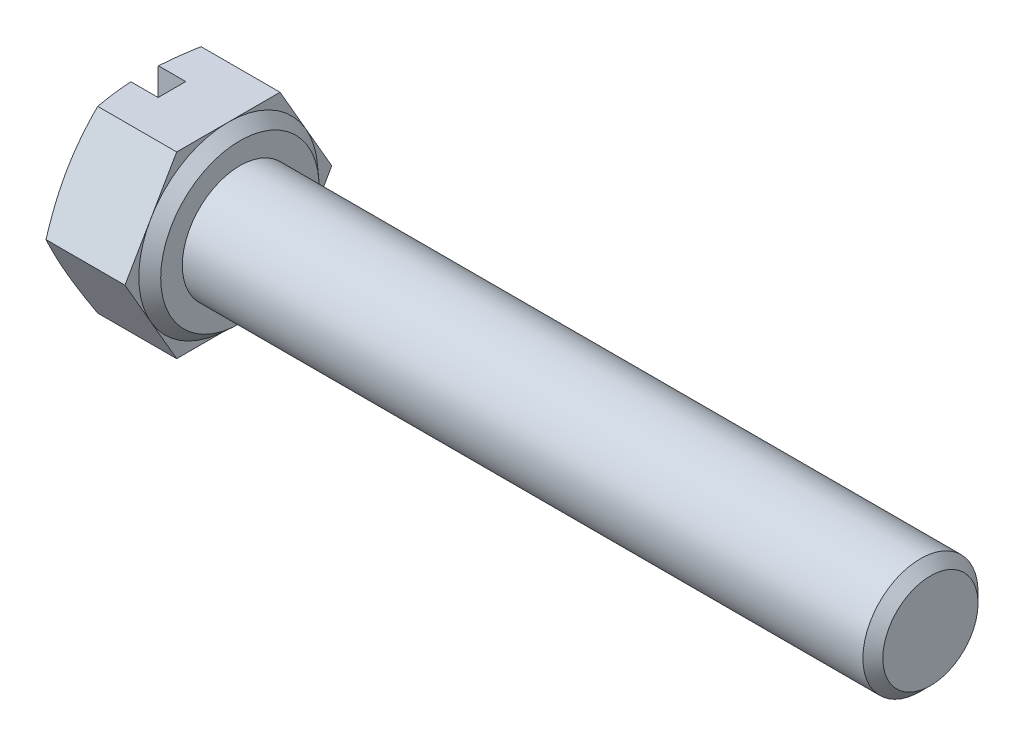
from build123d import *

# Parameters (mm, degrees)
BASEHEAD_DEPTH  = 3.65
SKETCH3_R       = 2.5
BASEBODY_DEPTH  = 30
CHAMFER1_SIZE   = 0.433
SLOT_DEPTH      = 35.663103343
SLOT_DEPTH_BACK = 35.663103343
SKETCH5_W       = 1.2
SKETCH5_H       = 1.2


with BuildPart() as part:
    # Sketch-BaseHead → BaseHead (new body)
    with BuildSketch(Plane(origin=(0, 0, 0), x_dir=(0, 0, -1), z_dir=(1, 0, 0))):
        Polygon((2.245892547, -3.89), (4.491785094, 0), (2.245892547, 3.89), (-2.245892547, 3.89), (-4.491785094, 0), (-2.245892547, -3.89), align=None)
    extrude(amount=BASEHEAD_DEPTH)

    # Sketch1 → Revolve1 (revolve)
    with BuildSketch(Plane.XY, mode=Mode.PRIVATE) as revolve1_sk:
        Polygon((3.65, 0), (4.15, 0), (4.15, -3.44), (3.65, -3.89), align=None)
    revolve(revolve1_sk.sketch.rotate(Axis((-4.001564945, 0, 0), (1, 0, 0)), 270), axis=Axis((-4.001564945, 0, 0), (1, 0, 0)))

    # Sketch3 → BaseBody (add)
    with BuildSketch(Plane(origin=(4.15, 0, 0), x_dir=(0, 0, -1), z_dir=(1, 0, 0))):
        Circle(SKETCH3_R)
    extrude(amount=BASEBODY_DEPTH)

    # Chamfer1
    chamfer1_edges = [part.edges().sort_by_distance(p)[0] for p in [
        (34.15, 0, 2.5),
    ]]
    chamfer(chamfer1_edges, length=CHAMFER1_SIZE)

    # Sketch4 → HeadChamfer (revolve, cut)
    with BuildSketch(Plane(origin=(-0.264637255, 0, 5.916896391), x_dir=(0, 0, -1), z_dir=(0, 1, 0)), mode=Mode.PRIVATE) as headchamfer_sk:
        Polygon((10.408681485, -0.264637255), (9.806896391, -0.264637255), (10.408681485, -0.483669117), align=None)
    revolve(headchamfer_sk.sketch.rotate(Axis((-4.001564945, 0, 0), (1, 0, 0)), 180), axis=Axis((-4.001564945, 0, 0), (1, 0, 0)), mode=Mode.SUBTRACT)

    # Sketch5 → Slot (cut, two sides: drawn at the far end of the back side and taken through both)
    with BuildSketch(Plane(origin=(0, 0, 0), x_dir=(1, 0, 0), z_dir=(0, 1, 0)).offset(-SLOT_DEPTH_BACK)):
        with Locations((0.6, 0)):
            Rectangle(SKETCH5_W, SKETCH5_H)
    extrude(amount=SLOT_DEPTH + SLOT_DEPTH_BACK, mode=Mode.SUBTRACT)


solid = part.part
